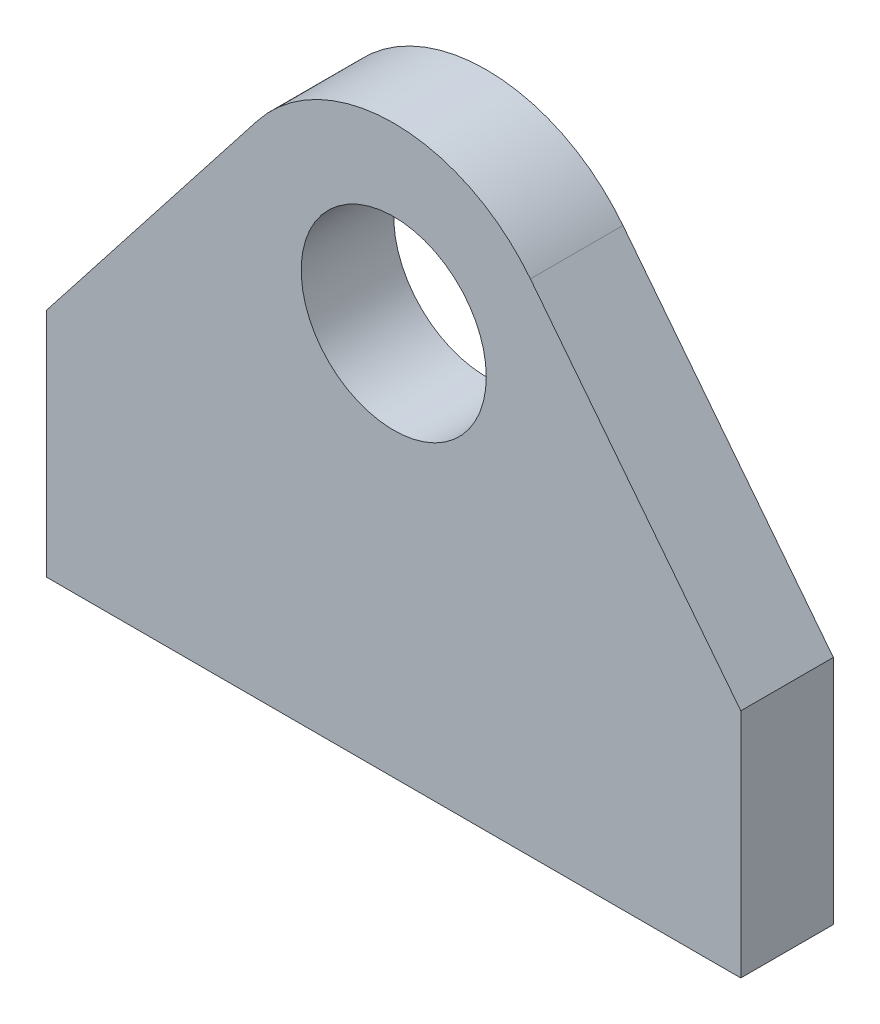
from build123d import *

# Parameters (mm, degrees)
SKETCH1_R           = 8
BOSS_EXTRUDE1_DEPTH = 8


with BuildPart() as part:
    # Sketch1 → Boss-Extrude1 (new body)
    with BuildSketch(Plane.XY):
        with BuildLine():
            Line((0, 0), (0, 20))
            Line((0, 20), (18.18643347, 43.243356849))
            ThreePointArc((18.18643347, 43.243356849), (30, 49), (41.81356653, 43.243356849))
            Line((41.81356653, 43.243356849), (60, 20))
            Line((60, 20), (60, 0))
            Line((60, 0), (0, 0))
        make_face()
        with Locations((30, 34)):
            Circle(SKETCH1_R, mode=Mode.SUBTRACT)
    extrude(amount=BOSS_EXTRUDE1_DEPTH)


solid = part.part
